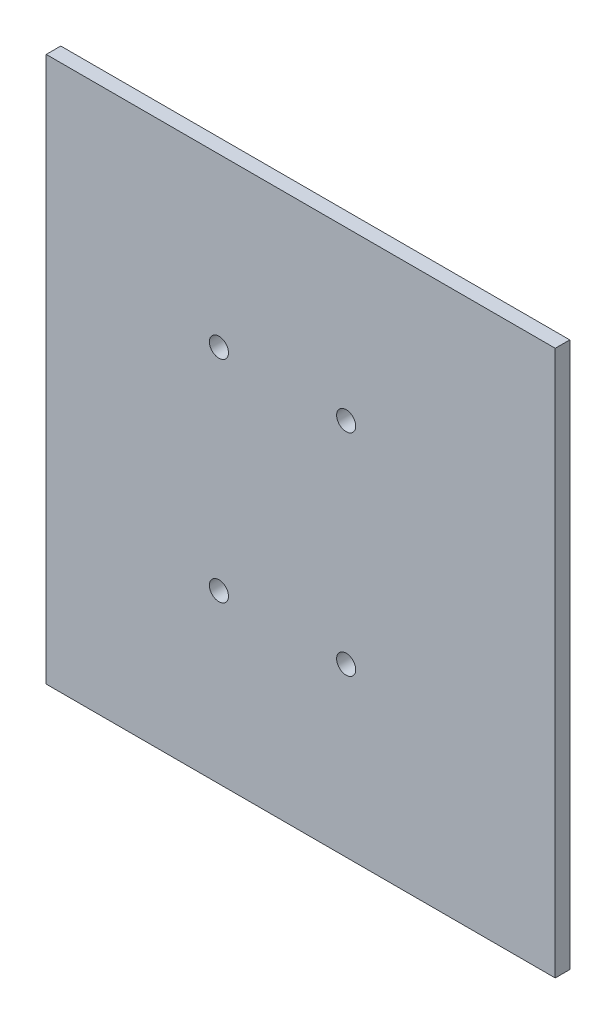
SolidWorks part; units mm, degrees
material "Q235B"
ref_plane "Front Plane" through (0, 0, 0) normal (0, 0, 1) x (1, 0, 0)
ref_plane "Top Plane" through (0, 0, 0) normal (0, 1, 0) x (1, 0, 0)
ref_plane "Right Plane" through (0, 0, 0) normal (1, 0, 0) x (0, 0, -1)
sketch "Sketch1" plane through (0, 0, 0) normal (0, 0, 1) x (1, 0, 0)
  line L1 (-81.6022, 41.8153) -> (198.3978, 41.8153)
  line L2 (-81.6022, 41.8153) -> (-81.6022, -258.1847)
  line L3 (-81.6022, -258.1847) -> (198.3978, -258.1847)
  line L4 (198.3978, 41.8153) -> (198.3978, -258.1847)
  dimension "D1" = 280
  dimension "D2" = 300
extrude "Boss-Extrude1" add sketch "Sketch1" along normal blind 8
sketch "Sketch2" plane through (0, 0, 0) normal (0, 0, -1) x (-1, 0, 0)
  line L0 (81.6022, -108.1847) -> (-198.3978, -108.1847) construction
  line L1 (81.6022, 41.8153) -> (81.6022, -258.1847) construction
  line L2 (-198.3978, -258.1847) -> (-198.3978, 41.8153) construction
  line L3 (-58.3978, -258.1847) -> (-58.3978, 41.8153) construction
  line L4 (81.6022, -258.1847) -> (-198.3978, -258.1847) construction
  line L5 (-198.3978, 41.8153) -> (81.6022, 41.8153) construction
  circle A0 centre (-13.3978, -50.1847) radius 5.25
  circle A1 centre (-83.3978, -50.1847) radius 5.25
  circle A2 centre (-13.3978, -166.1847) radius 5.25
  circle A3 centre (-83.3978, -166.1847) radius 5.25
  dimension "D1" = 10.5
  dimension "D4" = 25
  dimension "D2" = 70
  dimension "D3" = 58
extrude "Cut-Extrude1" cut sketch "Sketch2" against normal through all
